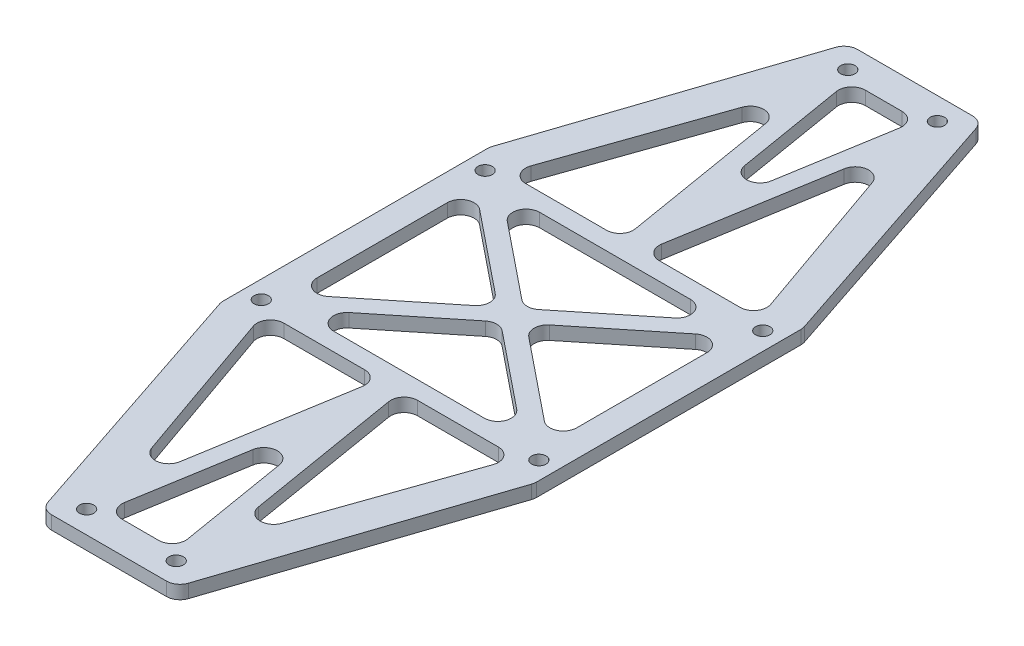
from build123d import *

# Parameters (mm, degrees)
EXTRUDE_1_DEPTH     = 3
SKETCH_2_R          = 1.6
CUT_EXTRUDE_1_DEPTH = 3
CUT_EXTRUDE_2_DEPTH = 3
FILLET_1_R          = 3


with BuildPart() as part:
    # 草图1 → 凸台-拉伸1 (new body)
    with BuildSketch(Plane(origin=(0, 0, 0), x_dir=(1, 0, 0), z_dir=(0, 1, 0))):
        Polygon((-15, 90), (-35, 30), (-35, -30), (-15, -90), (15, -90), (35, -30), (35, 30), (15, 90), align=None)
    extrude(amount=EXTRUDE_1_DEPTH)

    # 草图2 → 切除-拉伸1 (cut)
    with BuildSketch(Plane(origin=(0, 3, 0), x_dir=(1, 0, 0), z_dir=(0, 1, 0))):
        with Locations(Location((-31, 25, 0), (0, 0, 270))):
            Circle(SKETCH_2_R)
        with Locations(Location((31, 25, 0), (0, 0, 270))):
            Circle(SKETCH_2_R)
        with Locations(Location((31, -25, 0), (0, 0, 270))):
            Circle(SKETCH_2_R)
        with Locations(Location((-31, -25, 0), (0, 0, 270))):
            Circle(SKETCH_2_R)
        with Locations(Location((-10, 85, 0), (0, 0, 270))):
            Circle(SKETCH_2_R)
        with Locations(Location((10, 85, 0), (0, 0, 270))):
            Circle(SKETCH_2_R)
        with Locations(Location((10, -85, 0), (0, 0, 90))):
            Circle(SKETCH_2_R)
        with Locations(Location((-10, -85, 0), (0, 0, 90))):
            Circle(SKETCH_2_R)
    extrude(amount=-CUT_EXTRUDE_1_DEPTH, mode=Mode.SUBTRACT)

    # 草图4 → 切除-拉伸2 (cut)
    with BuildSketch(Plane(origin=(0, 3, 0), x_dir=(1, 0, 0), z_dir=(0, 1, 0))):
        Polygon((-10.689990891, 76.974420284), (-28.18103799, 27), (-2.360920843, 27), align=None)
        Polygon((10.689990891, 76.974420284), (2.360920843, 27), (28.18103799, 27), align=None)
        Polygon((7.639079157, 83), (-7.639079157, 83), (0, 37.165525061), align=None)
        Polygon((-1.694254177, 23), (-25.33403076, 23), (0, 2.569330032), (25.33403076, 23), (1.694254177, 23), (0, 12.834474939), align=None)
        Polygon((1.694254177, 23), (-1.694254177, 23), (0, 12.834474939), align=None)
        Polygon((-3.18596924, 0), (-29, 20.817766742), (-29, -20.817766742), align=None)
        Polygon((29, 20.817766742), (3.18596924, 0), (29, -20.817766742), align=None)
        Polygon((25.33403076, -23), (0, -2.569330032), (-25.33403076, -23), (-1.694254177, -23), (0, -12.834474939), (1.694254177, -23), align=None)
        Polygon((0, -12.834474939), (-1.694254177, -23), (1.694254177, -23), align=None)
        Polygon((-2.360920843, -27), (-28.18103799, -27), (-10.689990891, -76.974420284), align=None)
        Polygon((10.689990891, -76.974420284), (28.18103799, -27), (2.360920843, -27), align=None)
        Polygon((0, -37.165525061), (-7.639079157, -83), (7.639079157, -83), align=None)
    extrude(amount=-CUT_EXTRUDE_2_DEPTH, mode=Mode.SUBTRACT)

    # 圆角1
    fillet_1_edges = [part.edges().sort_by_distance(p)[0] for p in [
        (-28.18103799, 1.5, 27),
        (-2.360920843, 1.5, 27),
        (-10.689990891, 1.5, 76.974420284),
        (3.18596924, 1.5, 0),
        (29, 1.5, -20.817766742),
        (29, 1.5, 20.817766742),
        (-25.33403076, 1.5, 23),
        (0, 1.5, 2.569330032),
        (25.33403076, 1.5, 23),
        (25.33403076, 1.5, -23),
        (0, 1.5, -2.569330032),
        (-25.33403076, 1.5, -23),
        (-29, 1.5, 20.817766742),
        (-29, 1.5, -20.817766742),
        (-3.18596924, 1.5, 0),
        (2.360920843, 1.5, -27),
        (10.689990891, 1.5, -76.974420284),
        (28.18103799, 1.5, -27),
        (-7.639079157, 1.5, -83),
        (7.639079157, 1.5, -83),
        (0, 1.5, -37.165525061),
        (-7.639079157, 1.5, 83),
        (0, 1.5, 37.165525061),
        (7.639079157, 1.5, 83),
        (-28.18103799, 1.5, -27),
        (-10.689990891, 1.5, -76.974420284),
        (-2.360920843, 1.5, -27),
        (15, 1.5, -90),
        (35, 1.5, -30),
        (35, 1.5, 30),
        (15, 1.5, 90),
        (-15, 1.5, 90),
        (-35, 1.5, 30),
        (-35, 1.5, -30),
        (-15, 1.5, -90),
        (10.689990891, 1.5, 76.974420284),
        (2.360920843, 1.5, 27),
        (28.18103799, 1.5, 27),
    ]]
    fillet(fillet_1_edges, radius=FILLET_1_R)


solid = part.part
